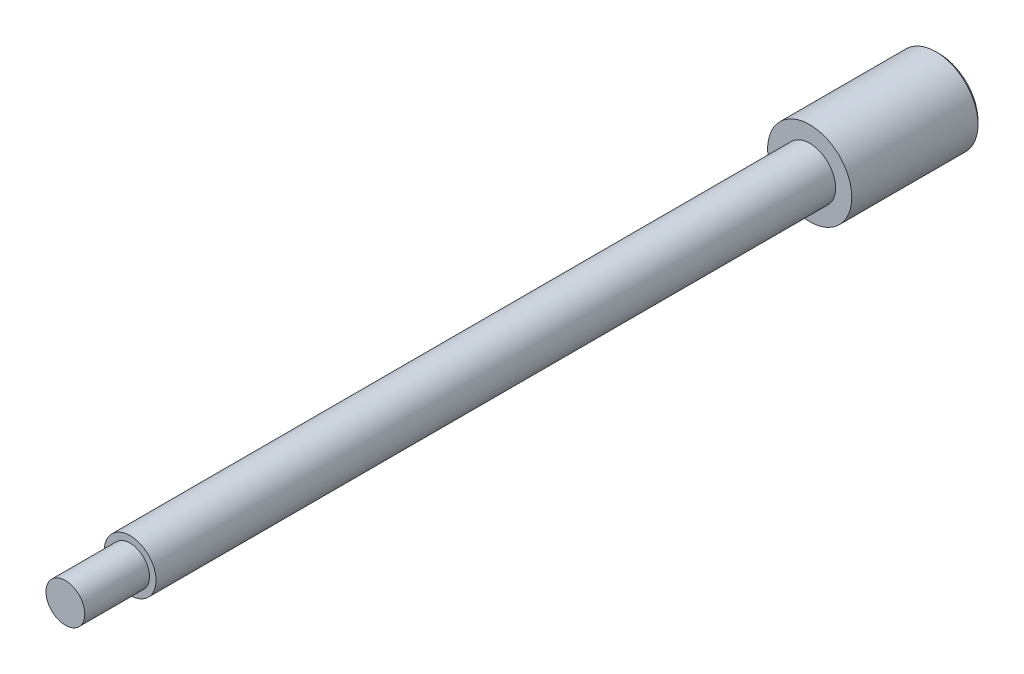
SolidWorks part; units mm, degrees
ref_plane "前视基准面" through (0, 0, 0) normal (0, 0, 1) x (1, 0, 0)
ref_plane "上视基准面" through (0, 0, 0) normal (0, 1, 0) x (1, 0, 0)
ref_plane "右视基准面" through (0, 0, 0) normal (1, 0, 0) x (0, 0, -1)
sketch "草图1" plane through (0, 0, 0) normal (0, 0, 1) x (1, 0, 0)
  circle A0 centre (0, 0) radius 6.5
  dimension "D1" = 13
extrude "凸台-拉伸1" add sketch "草图1" along normal blind 20
chamfer "倒角1" distance 0.5 angle 45 1 edges at (6.5, 0, 0)
hole_wizard "Ø2.0 (2) 直径孔1" positions "草图7" profile "草图6" hole size "Ø2.0" standard "GB"
sketch "草图7" plane through (0, 0, 0) normal (0, 0, -1) x (-1, 0, 0)
  line L0 (7.15, 0) -> (-7.15, 0) construction
  point P0 (-3.5, 0)
  point P2 (3.5, 0)
  dimension "D1" = 7
  dimension "D2" = 3.5
sketch "草图6" plane through (3.5, 0, 0) normal (1, 0, 0) x (0, 1, 0)
  line L0 (0, 0) -> (0, 5.6009)
  line L1 (0, 5.6009) -> (1, 5)
  line L2 (1, 5) -> (1, 0)
  line L5 (1, 0) -> (0, 0)
  line L10 (0, 5.6009) -> (-1, 5) construction
  line L11 (0, -6.35) -> (0, 107.95) construction
  dimension "孔直径" = 2
  dimension "孔深度" = 5
  dimension "导头角度" = 118
sketch "草图8" plane through (0, 0, 20) normal (0, 0, 1) x (1, 0, 0)
  circle A0 centre (0, 0) radius 4
  dimension "D1" = 8
extrude "凸台-拉伸2" add sketch "草图8" along normal blind 105
sketch "草图9" plane through (0, 0, 125) normal (0, 0, 1) x (1, 0, 0)
  circle A0 centre (0, 0) radius 3
  dimension "D1" = 6
extrude "凸台-拉伸3" add sketch "草图9" along normal blind 10
cosmetic thread "装饰螺纹线1" parameters "D2"=5
